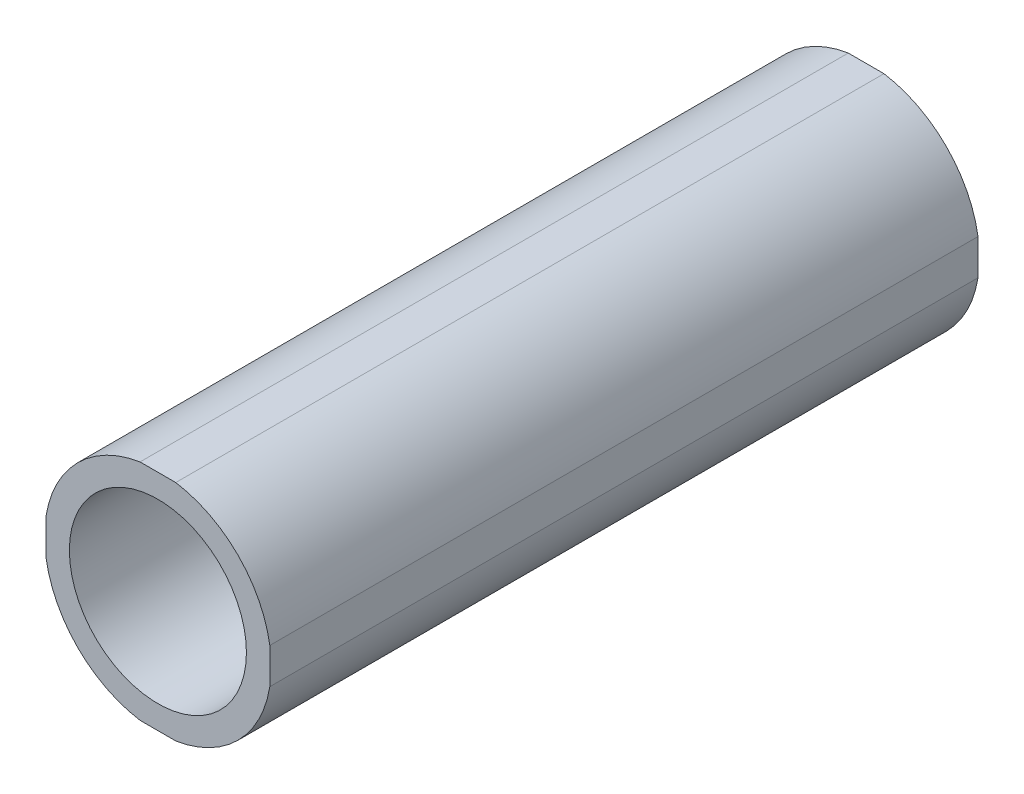
SolidWorks part; units mm, degrees
ref_plane "Front Plane" through (0, 0, 0) normal (0, 0, 1) x (1, 0, 0)
ref_plane "Top Plane" through (0, 0, 0) normal (0, 1, 0) x (1, 0, 0)
ref_plane "Right Plane" through (0, 0, 0) normal (1, 0, 0) x (0, 0, -1)
sketch "Sketch1" plane through (0, 0, 0) normal (0, 0, 1) x (1, 0, 0)
  circle A0 centre (0, 0) radius 8
  circle A1 centre (0, 0) radius 6.25
extrude "Boss-Extrude1" add sketch "Sketch1" along normal blind 50
sketch "Sketch2" plane through (0, 0, 50) normal (0, 0, 1) x (1, 0, 0)
  line L1 (7.9, 7.9) -> (-7.9, 7.9)
  line L2 (7.9, 7.9) -> (7.9, -7.9)
  line L3 (7.9, -7.9) -> (-7.9, -7.9)
  line L4 (-7.9, 7.9) -> (-7.9, -7.9)
  line L5 (7.9, 7.9) -> (-7.9, -7.9) construction
  line L6 (7.9, -7.9) -> (-7.9, 7.9) construction
  line L7 (10.4386, 10.0795) -> (-10.4386, 10.0795)
  line L8 (10.4386, 10.0795) -> (10.4386, -10.0795)
  line L9 (10.4386, -10.0795) -> (-10.4386, -10.0795)
  line L10 (-10.4386, 10.0795) -> (-10.4386, -10.0795)
  line L11 (10.4386, 10.0795) -> (-10.4386, -10.0795) construction
  line L12 (10.4386, -10.0795) -> (-10.4386, 10.0795) construction
  point P0 (0, 0)
  point P6 (0, 0)
  dimension "D1" = 15.8
  dimension "D2" = 15.8
extrude "Cut-Extrude1" cut sketch "Sketch2" against normal blind 50
